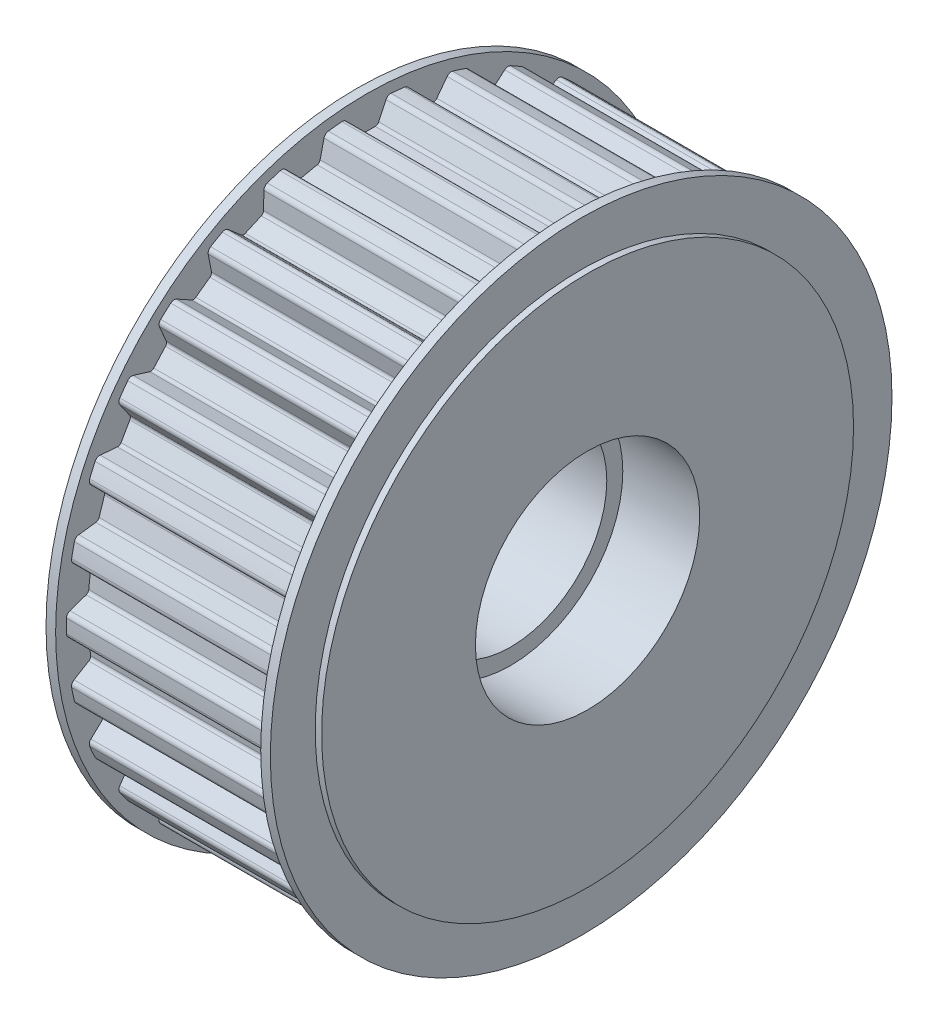
from build123d import *

# Parameters (mm, degrees)
SKETCH_1_R                       = 46.82
EXTRUDE_1_DEPTH                  = 16
CUT_EXTRUDE_2_DEPTH              = 32
FILLET_1_R                       = 0.6
FILLET_2_R                       = 0.8
PATTERN_CIRCULAR_1_COUNT         = 30
FILLET_1_OF_PATTERN_CIRCULAR_1_R = 0.6
FILLET_2_OF_PATTERN_CIRCULAR_1_R = 0.8
SKETCH_6_R                       = 48.5
EXTRUDE_2_DEPTH                  = 1.5
SKETCH_7_R                       = 41.5
EXTRUDE_3_DEPTH                  = 1
SKETCH_8_R                       = 15
CUT_EXTRUDE_1_DEPTH              = 78.932663242
SKETCH_9_R                       = 17.5
CUT_EXTRUDE_2_2_DEPTH            = 12


with BuildPart() as part:
    # 草图1 → 拉伸1 (new, symmetric)
    with BuildSketch(Plane(origin=(0, 0, 0), x_dir=(0, 0, -1), z_dir=(1, 0, 0))):
        Circle(SKETCH_1_R)
    extrude(amount=EXTRUDE_1_DEPTH, both=True)

    # 草图2 → Cut-Extrude 2 (cut)
    with BuildSketch(Plane(origin=(16, 0, 0), x_dir=(0, 0, -1), z_dir=(1, 0, 0))):
        with BuildLine():
            Line((-3.285, 46.704616207), (-1.753358309, 43.42))
            Line((-1.753358309, 43.42), (1.753358309, 43.42))
            Line((1.753358309, 43.42), (3.285, 46.704616207))
            ThreePointArc((3.285, 46.704616207), (0, 46.82), (-3.285, 46.704616207))
        make_face()
    cut_extrude_2 = extrude(amount=-CUT_EXTRUDE_2_DEPTH, mode=Mode.SUBTRACT)

    # 圆角1
    fillet_1_edges = [part.edges().sort_by_distance(p)[0] for p in [
        (0, 43.42, -1.753358309),
        (0, 43.42, 1.753358309),
    ]]
    fillet(fillet_1_edges, radius=FILLET_1_R)

    # 圆角2
    fillet_2_edges = [part.edges().sort_by_distance(p)[0] for p in [
        (0, 46.704616207, 3.285),
        (0, 46.704616207, -3.285),
    ]]
    fillet(fillet_2_edges, radius=FILLET_2_R)

    # 阵列(圆周)1: Cut-Extrude 2 ×30 about axis
    pattern_circular_1_axis = Axis((0, 0, 0), (1, 0, 0))
    for i in range(1, PATTERN_CIRCULAR_1_COUNT):
        add(cut_extrude_2.rotate(pattern_circular_1_axis, i * 360 / PATTERN_CIRCULAR_1_COUNT), mode=Mode.SUBTRACT)

    # 圆角1 of 阵列(圆周)1
    fillet_1_of_pattern_circular_1_edges = [part.edges().sort_by_distance(p)[0] for p in [
        (0, 42.835712514, 7.312482392),
        (0, 42.106625133, 10.742568838),
        (0, 40.379298843, 16.058732524),
        (0, 38.952988698, 19.262277561),
        (0, 36.158116052, 24.103138985),
        (0, 34.09691974, 26.940132324),
        (0, 30.356650082, 31.094122614),
        (0, 27.750651774, 33.440574031),
        (0, 23.228452837, 36.726143878),
        (0, 20.191547163, 38.479502187),
        (0, 15.085060741, 40.753056423),
        (0, 11.749975051, 41.836691452),
        (0, 6.282379104, 42.998864847),
        (0, 2.794872647, 43.365416546),
        (0, -2.794872647, 43.365416546),
        (0, -6.282379104, 42.998864847),
        (0, -11.749975051, 41.836691452),
        (0, -15.085060741, 40.753056423),
        (0, -20.191547163, 38.479502187),
        (0, -23.228452837, 36.726143878),
        (0, -27.750651774, 33.440574031),
        (0, -30.356650082, 31.094122614),
        (0, -34.09691974, 26.940132324),
        (0, -36.158116052, 24.103138985),
        (0, -38.952988698, 19.262277561),
        (0, -40.379298843, 16.058732524),
        (0, -42.106625133, 10.742568838),
        (0, -42.835712514, 7.312482392),
        (0, -43.42, 1.753358309),
        (0, -43.42, -1.753358309),
        (0, -42.835712514, -7.312482392),
        (0, -42.106625133, -10.742568838),
        (0, -40.379298843, -16.058732524),
        (0, -38.952988698, -19.262277561),
        (0, -36.158116052, -24.103138985),
        (0, -34.09691974, -26.940132324),
        (0, -30.356650082, -31.094122614),
        (0, -27.750651774, -33.440574031),
        (0, -23.228452837, -36.726143878),
        (0, -20.191547163, -38.479502187),
        (0, -15.085060741, -40.753056423),
        (0, -11.749975051, -41.836691452),
        (0, -6.282379104, -42.998864847),
        (0, -2.794872647, -43.365416546),
        (0, 2.794872647, -43.365416546),
        (0, 6.282379104, -42.998864847),
        (0, 11.749975051, -41.836691452),
        (0, 15.085060741, -40.753056423),
        (0, 20.191547163, -38.479502187),
        (0, 23.228452837, -36.726143878),
        (0, 27.750651774, -33.440574031),
        (0, 30.356650082, -31.094122614),
        (0, 34.09691974, -26.940132324),
        (0, 36.158116052, -24.103138985),
        (0, 38.952988698, -19.262277561),
        (0, 40.379298843, -16.058732524),
        (0, 42.106625133, -10.742568838),
        (0, 42.835712514, -7.312482392),
    ]]
    fillet(fillet_1_of_pattern_circular_1_edges, radius=FILLET_1_OF_PATTERN_CIRCULAR_1_R)

    # 圆角2 of 阵列(圆周)1
    fillet_2_of_pattern_circular_1_edges = [part.edges().sort_by_distance(p)[0] for p in [
        (0, 45.001018381, 12.923650593),
        (0, 46.36699819, 6.497220856),
        (0, 41.330660114, 21.99747564),
        (0, 44.002919859, 15.995481984),
        (0, 35.853953673, 30.109905447),
        (0, 39.715702781, 24.794663794),
        (0, 28.81025741, 36.906387902),
        (0, 33.692718914, 32.510199818),
        (0, 20.507414652, 42.089884109),
        (0, 26.197201555, 38.804884109),
        (0, 11.308299468, 45.433850411),
        (0, 17.55674078, 43.403608758),
        (0, 1.614957333, 46.792139434),
        (0, 8.148966186, 46.10538743),
        (0, -8.148966186, 46.10538743),
        (0, -1.614957333, 46.792139434),
        (0, -17.55674078, 43.403608758),
        (0, -11.308299468, 45.433850411),
        (0, -26.197201555, 38.804884109),
        (0, -20.507414652, 42.089884109),
        (0, -33.692718914, 32.510199818),
        (0, -28.81025741, 36.906387902),
        (0, -39.715702781, 24.794663794),
        (0, -35.853953673, 30.109905447),
        (0, -44.002919859, 15.995481984),
        (0, -41.330660114, 21.99747564),
        (0, -46.36699819, 6.497220856),
        (0, -45.001018381, 12.923650593),
        (0, -46.704616207, -3.285),
        (0, -46.704616207, 3.285),
        (0, -45.001018381, -12.923650593),
        (0, -46.36699819, -6.497220856),
        (0, -41.330660114, -21.99747564),
        (0, -44.002919859, -15.995481984),
        (0, -35.853953673, -30.109905447),
        (0, -39.715702781, -24.794663794),
        (0, -28.81025741, -36.906387902),
        (0, -33.692718914, -32.510199818),
        (0, -20.507414652, -42.089884109),
        (0, -26.197201555, -38.804884109),
        (0, -11.308299468, -45.433850411),
        (0, -17.55674078, -43.403608758),
        (0, -1.614957333, -46.792139434),
        (0, -8.148966186, -46.10538743),
        (0, 8.148966186, -46.10538743),
        (0, 1.614957333, -46.792139434),
        (0, 17.55674078, -43.403608758),
        (0, 11.308299468, -45.433850411),
        (0, 26.197201555, -38.804884109),
        (0, 20.507414652, -42.089884109),
        (0, 33.692718914, -32.510199818),
        (0, 28.81025741, -36.906387902),
        (0, 39.715702781, -24.794663794),
        (0, 35.853953673, -30.109905447),
        (0, 44.002919859, -15.995481984),
        (0, 41.330660114, -21.99747564),
        (0, 46.36699819, -6.497220856),
        (0, 45.001018381, -12.923650593),
    ]]
    fillet(fillet_2_of_pattern_circular_1_edges, radius=FILLET_2_OF_PATTERN_CIRCULAR_1_R)

    # 草图6 → 凸台-拉伸2 (add)
    with BuildSketch(Plane(origin=(16, 0, 0), x_dir=(0, 0, -1), z_dir=(1, 0, 0))):
        Circle(SKETCH_6_R)
    extrude_2 = extrude(amount=EXTRUDE_2_DEPTH)

    # 草图7 → 凸台-拉伸3 (add)
    with BuildSketch(Plane(origin=(17.5, 0, 0), x_dir=(0, 0, -1), z_dir=(1, 0, 0))):
        Circle(SKETCH_7_R)
    extrude_3 = extrude(amount=EXTRUDE_3_DEPTH)

    # 镜向2: 凸台-拉伸2, 凸台-拉伸3 across plane
    add(extrude_2.mirror(Plane(origin=(0, 0, 0), x_dir=(0, 0, 1), z_dir=(1, 0, 0))))
    add(extrude_3.mirror(Plane(origin=(0, 0, 0), x_dir=(0, 0, 1), z_dir=(1, 0, 0))))

    # 草图8 → 切除-拉伸1 (cut, through all)
    with BuildSketch(Plane.ZY.offset(18.5)):
        Circle(SKETCH_8_R)
    extrude(amount=-CUT_EXTRUDE_1_DEPTH, mode=Mode.SUBTRACT)

    # 草图9 → Cut-Extrude 2 2 (cut)
    with BuildSketch(Plane.ZY.offset(18.5)):
        Circle(SKETCH_9_R)
    cut_extrude_2_2 = extrude(amount=-CUT_EXTRUDE_2_2_DEPTH, mode=Mode.SUBTRACT)

    # 镜向3: Cut-Extrude 2 2 across plane
    add(cut_extrude_2_2.mirror(Plane(origin=(0, 0, 0), x_dir=(0, 0, 1), z_dir=(1, 0, 0))), mode=Mode.SUBTRACT)


solid = part.part
